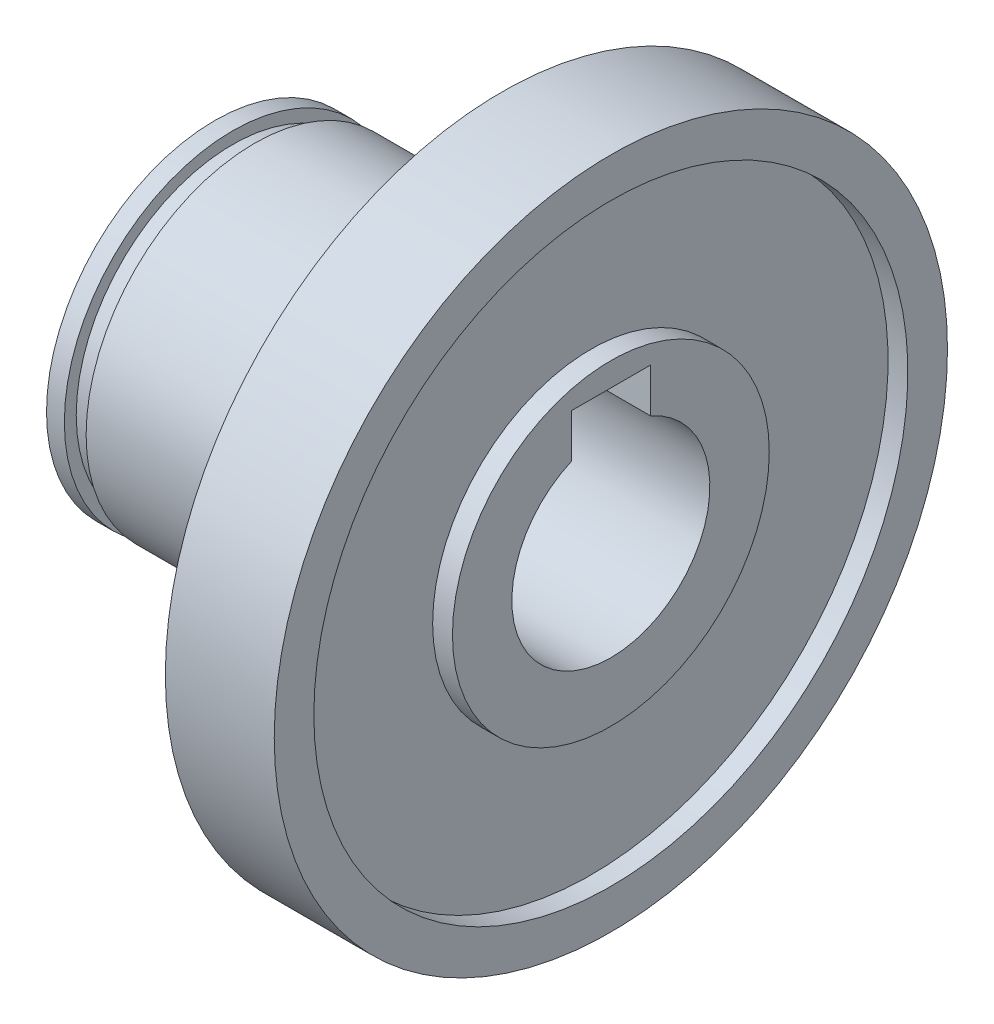
SolidWorks part; units mm, degrees
ref_plane "前视基准面" through (0, 0, 0) normal (0, 0, 1) x (1, 0, 0)
ref_plane "上视基准面" through (0, 0, 0) normal (0, 1, 0) x (1, 0, 0)
ref_plane "右视基准面" through (0, 0, 0) normal (1, 0, 0) x (0, 0, -1)
sketch "草图1" plane through (0, 0, 0) normal (0, 0, 1) x (1, 0, 0)
  line L0 (0, 0) -> (60.054, 0) construction
  line L1 (0, 5) -> (20, 5)
  line L2 (20, 5) -> (20, 8)
  line L3 (20, 8) -> (19, 8)
  line L4 (19, 8) -> (19, 15)
  line L5 (19, 15) -> (20, 15)
  line L6 (20, 15) -> (20, 17)
  line L7 (20, 17) -> (14.5, 17)
  line L8 (14.5, 17) -> (14.5, 8.5)
  line L9 (14.5, 8.5) -> (2, 8.5)
  line L10 (2, 8.5) -> (2, 7.9)
  line L11 (2, 7.9) -> (0.9, 7.9)
  line L12 (0.9, 7.9) -> (0.9, 8.5)
  line L13 (0.9, 8.5) -> (0, 8.5)
  line L14 (0, 8.5) -> (0, 5)
  dimension "D1" = 5
  dimension "D2" = 20
  dimension "D3" = 3
  dimension "D4" = 1
  dimension "D5" = 7
  dimension "D6" = 1
  dimension "D7" = 2
  dimension "D8" = 5.5
  dimension "D9" = 8.5
  dimension "D10" = 12.5
  dimension "D11" = 1.1
  dimension "D12" = 3.5
  dimension "D13" = 0.6
revolve "旋转1" add sketch "草图1" angle 360 about L0
sketch "草图2" plane through (20, 0, 0) normal (1, 0, 0) x (0, 0, -1)
  line L1 (-2, 0) -> (2, 0)
  line L2 (-2, 0) -> (-2, 6.8)
  line L3 (-2, 6.8) -> (2, 6.8)
  line L4 (2, 0) -> (2, 6.8)
  dimension "D1" = 4
  dimension "D2" = 2
  dimension "D3" = 6.8
extrude "切除-拉伸1" cut sketch "草图2" against normal through all
